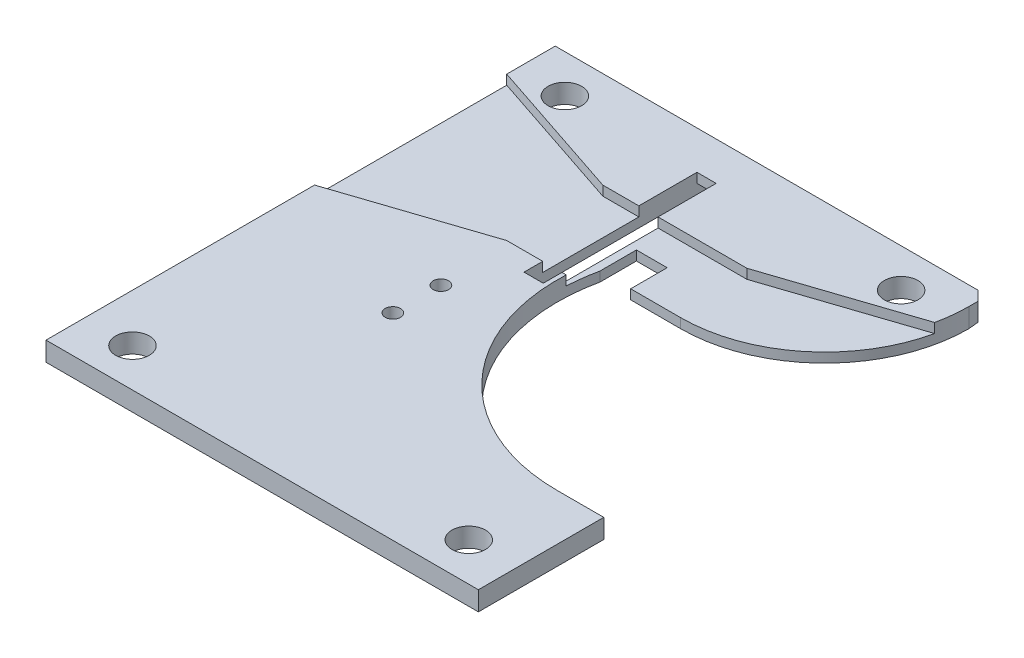
from build123d import *
from OCP.BRepFilletAPI import BRepFilletAPI_MakeChamfer

# Parameters (mm, degrees)
SKETCH1_W             = 45
SKETCH1_H             = 50
BOSS_EXTRUDE1_DEPTH   = 2
SKETCH2_W             = 3.2
SKETCH2_H             = 3.8
CUT_EXTRUDE1_DEPTH    = 34.693471178
SKETCH3_W             = 2
SKETCH3_H             = 18
CUT_EXTRUDE2_DEPTH    = 34.693471178
SKETCH4_W             = 2
SKETCH4_H             = 4
CUT_EXTRUDE3_DEPTH    = 1
CUT_EXTRUDE4_DEPTH    = 3
SKETCH6_W             = 46.8
SKETCH6_H             = 10
CUT_EXTRUDE5_DEPTH    = 1
CHAMFER1_SIZE         = 15
CHAMFER1_SIZE2        = 5
CHAMFER2_SIZE         = 5
CHAMFER2_SIZE2        = 15
SKETCH8_W             = 45
SKETCH8_H             = 2
BOSS_EXTRUDE2_DEPTH   = 3
SKETCH7_R             = 1.75
CUT_EXTRUDE6_DEPTH    = 36.975686234
FILLET2_R             = 15
CHAMFER4_SIZE         = 2
CHAMFER4_SIZE2        = 0.2
SKETCH10_W            = 4.825824379
SKETCH10_H            = 2.951447422
CUT_EXTRUDE7_DEPTH    = 36.975686234
CHAMFER5_SIZE         = 1
M2_TAPPED_HOLE1_D     = 1.6
M2_TAPPED_HOLE1_DEPTH = 5.2
M2_TAPPED_HOLE1_TIP   = 0.480688495


with BuildPart() as part:
    # Sketch1 → Boss-Extrude1 (new body)
    with BuildSketch(Plane(origin=(0, 0, 0), x_dir=(1, 0, 0), z_dir=(0, 1, 0))):
        Rectangle(SKETCH1_W, SKETCH1_H)
    extrude(amount=BOSS_EXTRUDE1_DEPTH)

    # Sketch2 → Cut-Extrude1 (cut, through all)
    with BuildSketch(Plane(origin=(0, 2, 0), x_dir=(1, 0, 0), z_dir=(0, 1, 0))):
        with Locations((0.7, 9.95)):
            Rectangle(SKETCH2_W, SKETCH2_H)
    extrude(amount=-CUT_EXTRUDE1_DEPTH, mode=Mode.SUBTRACT)

    # Sketch3 → Cut-Extrude2 (cut, through all)
    with BuildSketch(Plane(origin=(0, 2, 0), x_dir=(1, 0, 0), z_dir=(0, 1, 0))):
        with Locations((-2.75, 12)):
            Rectangle(SKETCH3_W, SKETCH3_H)
    extrude(amount=-CUT_EXTRUDE2_DEPTH, mode=Mode.SUBTRACT)

    # Sketch4 → Cut-Extrude3 (cut)
    with BuildSketch(Plane.XZ):
        with Locations((-2.75, -23)):
            Rectangle(SKETCH4_W, SKETCH4_H)
    extrude(amount=-CUT_EXTRUDE3_DEPTH, mode=Mode.SUBTRACT)

    # Sketch5 → Cut-Extrude4 (cut)
    with BuildSketch(Plane(origin=(0, 2, 0), x_dir=(1, 0, 0), z_dir=(0, 1, 0))):
        with BuildLine():
            Line((-0.9, 8.05), (26.461433113, 8.05))
            Line((26.461433113, 8.05), (36.248351242, 8.05))
            ThreePointArc((36.248351242, 8.05), (17.674175621, -14.95), (-0.9, 8.05))
        make_face()
    extrude(amount=-CUT_EXTRUDE4_DEPTH, mode=Mode.SUBTRACT)

    # Sketch6 → Cut-Extrude5 (cut)
    with BuildSketch(Plane(origin=(0, 2, 0), x_dir=(1, 0, 0), z_dir=(0, 1, 0))):
        with Locations((-0.9, 9.95)):
            Rectangle(SKETCH6_W, SKETCH6_H)
    extrude(amount=-CUT_EXTRUDE5_DEPTH, mode=Mode.SUBTRACT)

    # Chamfer1: one chamfer whose edges measure the first distance from different faces: ONE call of the kernel's chamfer builder (chamfer() names one face for all edges)
    chamfer1_edges_1 = [part.edges().sort_by_distance(p)[0] for p in [
        (-22.5, 1.5, -14.95),
    ]]
    chamfer1_side_1 = [part.faces().sort_by_distance(p)[0] for p in [
        (-13.125, 1.5, -14.95),
    ]]
    chamfer1_edges_2 = [part.edges().sort_by_distance(p)[0] for p in [
        (-22.5, 1.5, -4.95),
    ]]
    chamfer1_side_2 = [part.faces().sort_by_distance(p)[0] for p in [
        (-13.125, 1.5, -4.95),
    ]]
    chamfer1 = BRepFilletAPI_MakeChamfer(part.part.solid().wrapped)
    for e in chamfer1_edges_1:
        chamfer1.Add(CHAMFER1_SIZE, CHAMFER1_SIZE2, e.wrapped, chamfer1_side_1[0].wrapped)  # the first distance lies on this face
    for e in chamfer1_edges_2:
        chamfer1.Add(CHAMFER1_SIZE, CHAMFER1_SIZE2, e.wrapped, chamfer1_side_2[0].wrapped)  # the first distance lies on this face
    add(Compound.cast(chamfer1.Shape()), mode=Mode.REPLACE)

    # Chamfer2
    chamfer2_edges = [part.edges().sort_by_distance(p)[0] for p in [
        (22.5, 1.5, -14.95),
    ]]
    chamfer2_side = [part.faces().sort_by_distance(p)[0] for p in [
        (22.5, 0.872222222, -17.809166667),
    ]]
    chamfer(chamfer2_edges, length=CHAMFER2_SIZE, length2=CHAMFER2_SIZE2, reference=chamfer2_side[0])

    # Sketch8 → Boss-Extrude2 (add)
    with BuildSketch(Plane.XY.offset(25)):
        with Locations((0, 1)):
            Rectangle(SKETCH8_W, SKETCH8_H)
    extrude(amount=BOSS_EXTRUDE2_DEPTH)

    # Sketch7 → Cut-Extrude6 (cut, through all)
    with BuildSketch(Plane(origin=(0, 2, 0), x_dir=(1, 0, 0), z_dir=(0, 1, 0))):
        with Locations(Location((-17.5, 21, 0), (0, 0, 270))):
            Circle(SKETCH7_R)
        with Locations(Location((17.5, 21, 0), (0, 0, 90))):
            Circle(SKETCH7_R)
        with Locations(Location((17.5, -24, 0), (0, 0, 270))):
            Circle(SKETCH7_R)
        with Locations(Location((-17.5, -24, 0), (0, 0, 90))):
            Circle(SKETCH7_R)
    extrude(amount=-CUT_EXTRUDE6_DEPTH, mode=Mode.SUBTRACT)

    # Fillet2
    fillet2_edges = [part.edges().sort_by_distance(p)[0] for p in [
        (22.5, 0.5, -8.05),
    ]]
    fillet(fillet2_edges, radius=FILLET2_R)

    # Chamfer4
    chamfer4_edges = [part.edges().sort_by_distance(p)[0] for p in [
        (10.375, 0, -25),
        (-13.125, 0, -25),
    ]]
    chamfer4_side = [part.faces().sort_by_distance(p)[0] for p in [
        (-3.590988943, 0, 2.118757262),
    ]]
    chamfer(chamfer4_edges, length=CHAMFER4_SIZE, length2=CHAMFER4_SIZE2, reference=chamfer4_side[0])

    # Sketch10 → Cut-Extrude7 (cut, through all)
    with BuildSketch(Plane(origin=(0, 2, 0), x_dir=(1, 0, 0), z_dir=(0, 1, 0))):
        with Locations((20.087087811, -13.474276289)):
            Rectangle(SKETCH10_W, SKETCH10_H)
    extrude(amount=-CUT_EXTRUDE7_DEPTH, mode=Mode.SUBTRACT)

    # Chamfer5
    chamfer5_edges = [part.edges().sort_by_distance(p)[0] for p in [
        (22.5, 1.1, -25),
    ]]
    chamfer(chamfer5_edges, length=CHAMFER5_SIZE)

    # M2 Tapped Hole1
    with Locations(Plane(origin=(0, 2, 0), x_dir=(1, 0, 0), z_dir=(0, 1, 0))):
        with Locations((-6.9, -7.5), (-6.9, -2.5)):
            Hole(M2_TAPPED_HOLE1_D / 2, depth=M2_TAPPED_HOLE1_DEPTH)
            with Locations((0, 0, -(M2_TAPPED_HOLE1_DEPTH + M2_TAPPED_HOLE1_TIP / 2))):  # 118° drill point
                Cone(0, M2_TAPPED_HOLE1_D / 2, M2_TAPPED_HOLE1_TIP, mode=Mode.SUBTRACT)


solid = part.part
